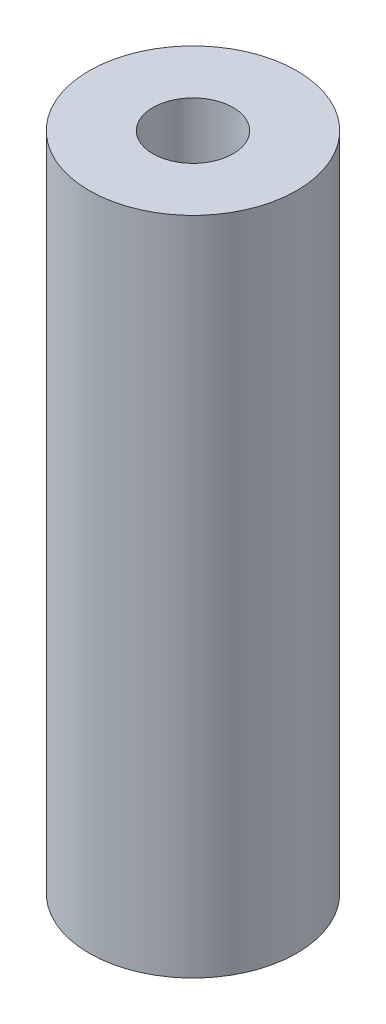
SolidWorks part; units mm, degrees
material "SS400B"
ref_plane "Front Plane" through (0, 0, 0) normal (0, 0, 1) x (1, 0, 0)
ref_plane "Top Plane" through (0, 0, 0) normal (0, 1, 0) x (1, 0, 0)
ref_plane "Right Plane" through (0, 0, 0) normal (1, 0, 0) x (0, 0, -1)
sketch "Sketch1" plane through (0, 0, 0) normal (0, 1, 0) x (1, 0, 0)
  circle A0 centre (0, 0) radius 11
  dimension "D1" = 22
extrude "Boss-Extrude1" add sketch "Sketch1" along normal blind 70
hole_wizard "M10 Tapped Hole1" positions "Sketch2" profile "Sketch3" tap size "M10" standard "GB"
sketch "Sketch2" plane through (0, 70, 0) normal (0, 1, 0) x (1, 0, 0)
  point P0 (0, 0)
sketch "Sketch3" plane through (0, 70, 0) normal (1, 0, 0) x (0, 0, 1)
  line L0 (0, 0) -> (0, 27.5537)
  line L1 (0, 27.5537) -> (4.25, 25)
  line L2 (4.25, 25) -> (4.25, 0)
  line L5 (4.25, 0) -> (0, 0)
  line L10 (0, 27.5537) -> (-4.25, 25) construction
  line L11 (0, -6.35) -> (0, 107.95) construction
  dimension "螺纹孔钻头直径" = 8.5
  dimension "螺纹孔钻头深度" = 25
  dimension "导头角度" = 118
cosmetic thread "Cosmetic Thread1"
